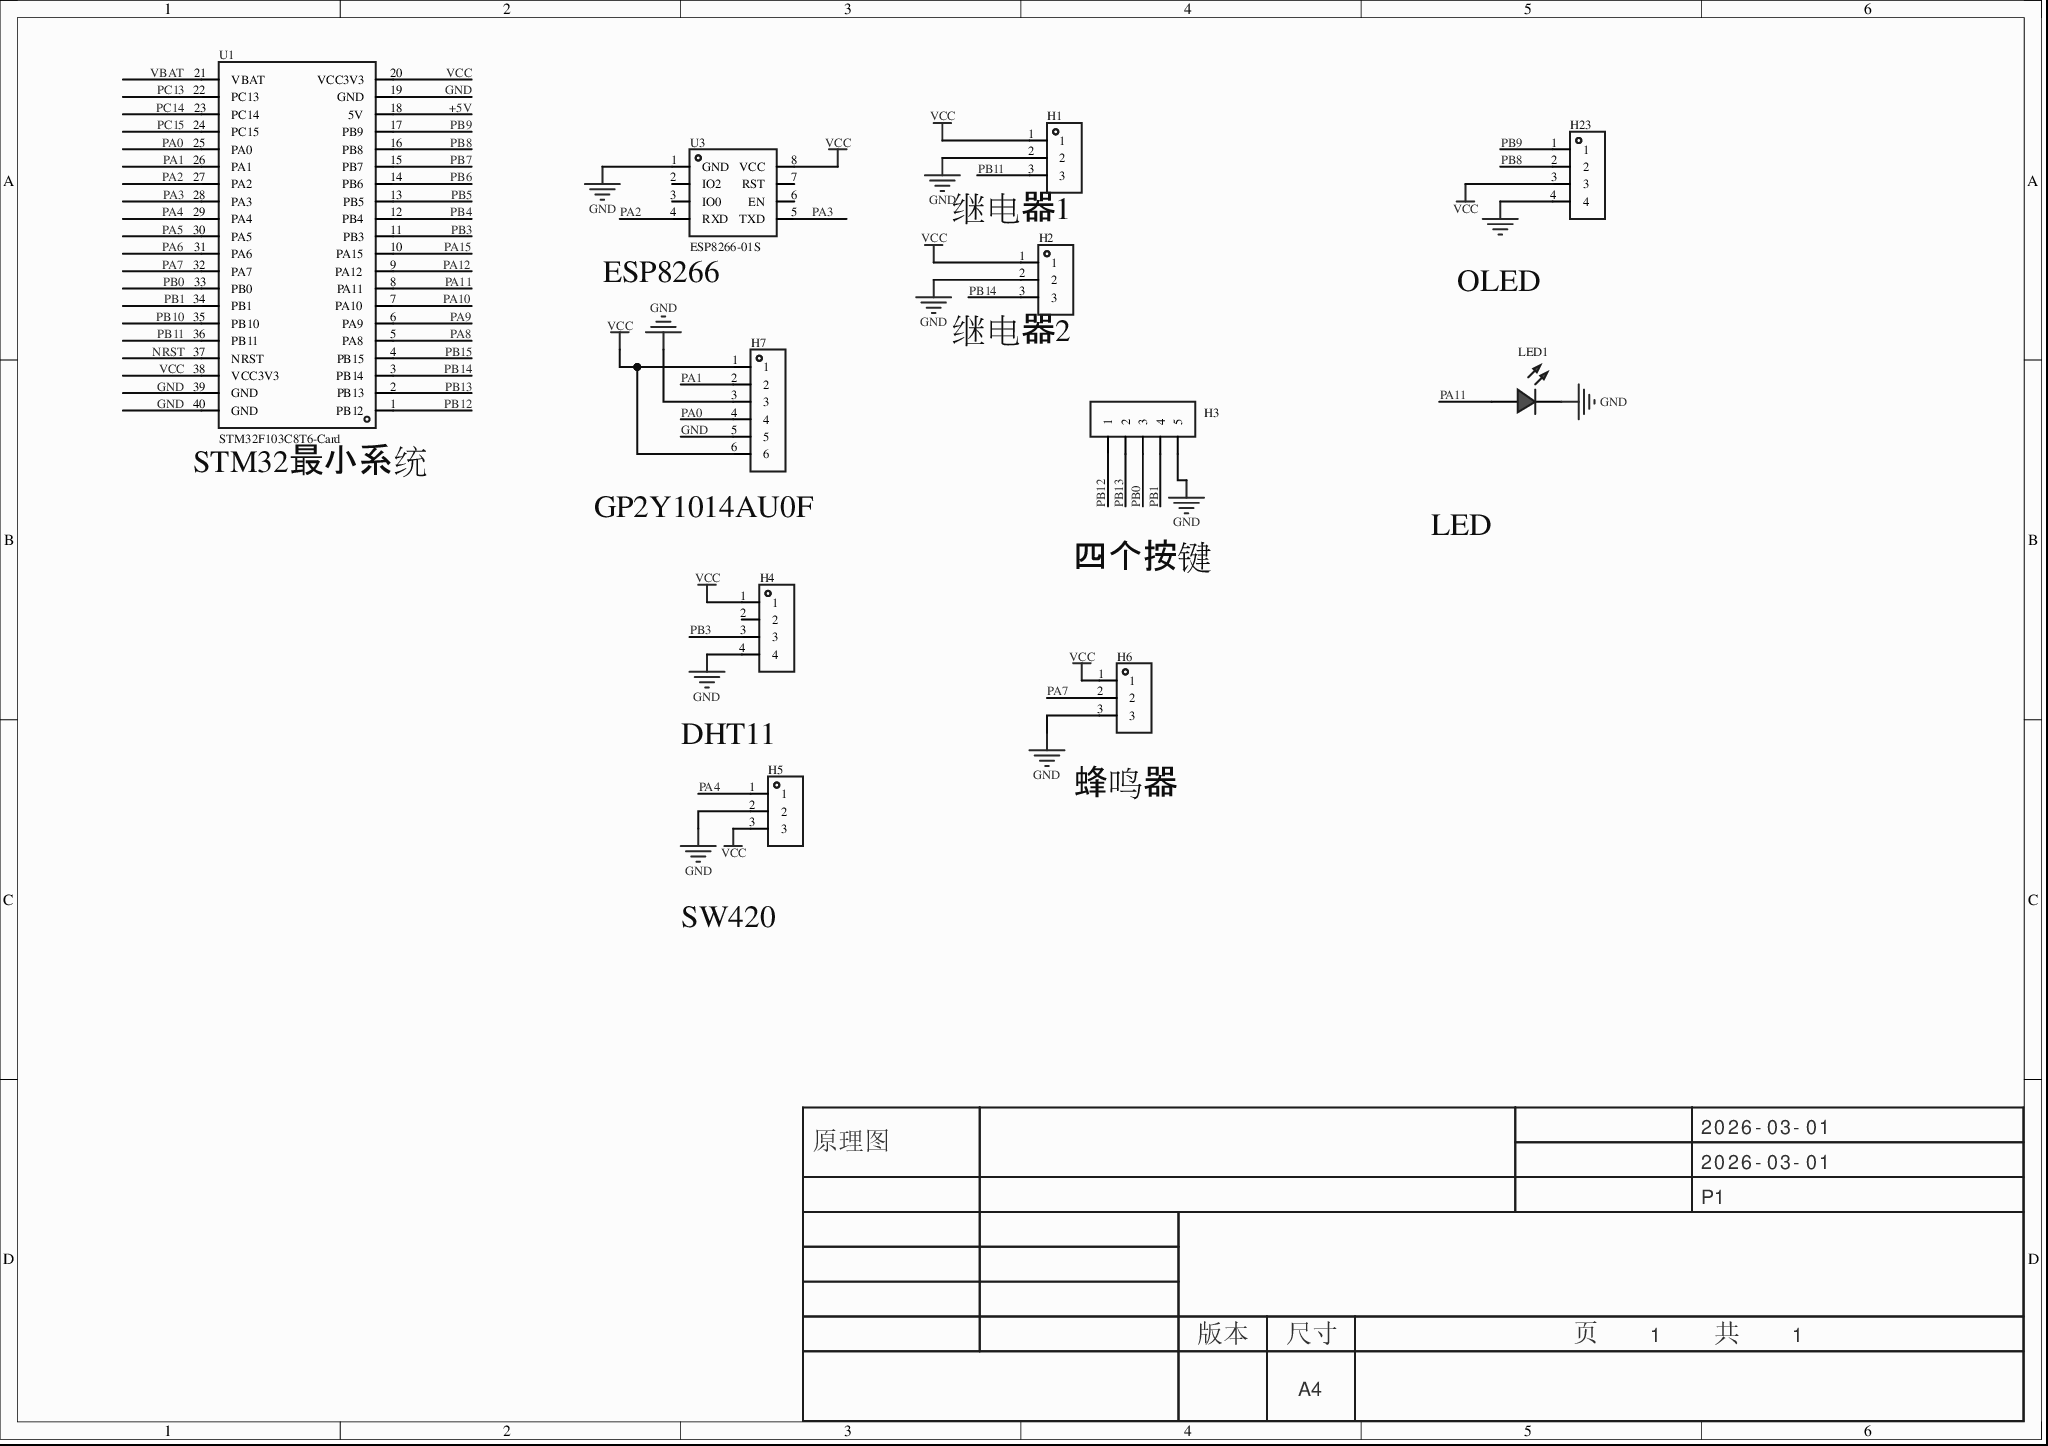
[diagram p0: MISC51358-3.schdoc]
# Altium project MISC51358-2.PrjPcb
1 sheet, 11 parts. Net scope: global (net labels, ports and power ports of the same name join across sheets).
Board file: MISC51358.pcbdoc

## Sheet MISC51358-3.schdoc
size 297 x 209 mm; Version: V1.0; @Project Name: MISC51358; @Page Count: 1; @Update Date: 2026-03-01; @Create Date: 2026-03-01; @Schematic Name: MISC51358; @Page No: 1; @Create Time: 18:58:15; @Update Time: 22:44:58; @Board Name: MISC51358

### Parts
H1  (no value)  [HDR-TH_3P-P2.54-V-F]
H2  (no value)  [HDR-TH_3P-P2.54-V-F]
H3  (no value)  [HDR-TH_5P-P2.54-V-F]
H4  (no value)  [HDR-TH_4P-P2.54-V-F]
H5  (no value)  [HDR-TH_3P-P2.54-V-F]
H6  (no value)  [HDR-TH_3P-P2.54-V-F]
H7  (no value)  [HDR-TH_6P-P2.54-V-F]
H23  (no value)  [HDR-TH_4P-P2.54-V-F]
LED1  (no value)  [LED_TH-3mm]
U1  STM32F103C8T6-Card  [CONN-TH_L53.3-W22.9_STM32F103C8T6-CARD]
U3  ESP8266-01S  [WIFIM-TH_ESP8266-01S]

### Nets
GND: H1.2 H2.2 H3.5 H4.4 H5.2 H6.3 H7.3 H7.5 H23.4 LED1.2(A) U1.19(GND) U1.39(GND) U1.40(GND) U3.1(GND)
VCC: H1.1 H2.1 H4.1 H5.3 H6.1 H7.1 H7.6 H23.3 U1.20(VCC3V3) U1.38(VCC3V3) U3.8(VCC)
+5V: U1.18(5V)
NRST: U1.37(NRST)
PA0: H7.4 U1.25(PA0)
PA1: H7.2 U1.26(PA1)
PA2: U1.27(PA2) U3.4(RXD)
PA3: U1.28(PA3) U3.5(TXD)
PA4: H5.1 U1.29(PA4)
PA5: U1.30(PA5)
PA6: U1.31(PA6)
PA7: H6.2 U1.32(PA7)
PA8: U1.5(PA8)
PA9: U1.6(PA9)
PA10: U1.7(PA10)
PA11: LED1.1(C) U1.8(PA11)
PA12: U1.9(PA12)
PA15: U1.10(PA15)
PB0: H3.3 U1.33(PB0)
PB1: H3.4 U1.34(PB1)
PB3: H4.3 U1.11(PB3)
PB4: U1.12(PB4)
PB5: U1.13(PB5)
PB6: U1.14(PB6)
PB7: U1.15(PB7)
PB8: H23.2 U1.16(PB8)
PB9: H23.1 U1.17(PB9)
PB10: U1.35(PB10)
PB11: H1.3 U1.36(PB11)
PB12: H3.1 U1.1(PB12)
PB13: H3.2 U1.2(PB13)
PB14: H2.3 U1.3(PB14)
PB15: U1.4(PB15)
PC13: U1.22(PC13)
PC14: U1.23(PC14)
PC15: U1.24(PC15)
VBAT: U1.21(VBAT)

Not connected (* = marked no-connect by the designer): H4 2*; U3 2(IO2) 3(IO0) 6(EN) 7(RST)

### Notes on the sheet
- 继电器1
- (near U3) ESP8266
- (near H2) 继电器2
- OLED
- (near U1) STM32最小系统
- (near H7) GP2Y1014AU0F
- 四个按键
- LED
- DHT11
- (near H6) 蜂鸣器
- SW420
- 2026-03-01
- 原理图
- P1
- 版本
- 尺寸
- A4
- 页    1    共    1

### Library data of the parts
H1 H2 H5 H6 = HDR-F_2.54_1x3P: Symbol: PM254V-11-03-H85; 3D Model: f3b3cc5aae9641bf9e56fc160cef875b; 3D Model Transform: 299.9994,100,0,0,0,0,0,0,-118.11; ConvertToPcb: yes; ModelName: HDR2.54-F-LI-1X3P; Device: HDR-F_2.54_1x3P; Supplier Part: C541850; Supplier Footprint: 插件; AddInBom: yes; FootprintName: HDR-TH_3P-P2.54-V-F
H3 = HDR-F_2.54_1x5P: Symbol: Header-Female-2.54_1x5; ConvertToPcb: yes; ModelId: f49cb6116a3d45e5a64915bf3e00773f; ModelTransform: 519.684,98.464,0,0,0,0,0,0,-124.016; Device: HDR-F_2.54_1x5P; AddInBom: yes; SupplierPart: C50950; Supplier Footprint: 插件; FootprintName: HDR-TH_5P-P2.54-V-F; ModelName: HDR-TH_5P-P2.54-V-F
H4 = HDR-F_2.54_1x4P: Symbol: 2.54-1*4P母; ConvertToPcb: yes; ModelId: d187812051054f85879fcaa51a310d8e0819f05c4eef4c71ace90d822a990e87; ModelTransform: 419.6842,98.464,0,0,0,0,0,0,-118.11; Device: HDR-F_2.54_1x4P; AddInBom: yes; SupplierPart: C2718488; Supplier Footprint: 插件; FootprintName: HDR-TH_4P-P2.54-V-F; ModelName: HDR-TH_4P-P2.54-V-F
H7 = HDR-F_2.54_1x6P: Symbol: Header-Female-2.54_1x6; 3D Model: 0f5bcf94dcda47d085f24cdca1696fe9; 3D Model Transform: 619.684,94.488,0,0,0,0,0,0,-125.984; ConvertToPcb: yes; Device: HDR-F_2.54_1x6P; Supplier Part: C40877; Supplier Footprint: 插件; AddInBom: yes; FootprintName: HDR-TH_6P-P2.54-V-F; ModelName: HDR-TH_6P-P2.54-V-F
H23 = HDR-F_2.54_1x4P: Symbol: 2.54-1*4P母; ConvertToPcb: yes; ModelId: d187812051054f85879fcaa51a310d8e; ModelTransform: 419.6842,98.464,0,0,0,0,0,0,-118.11; Device: HDR-F_2.54_1x4P; AddInBom: yes; SupplierPart: C2718488; Supplier Footprint: 插件; FootprintName: HDR-TH_4P-P2.54-V-F; ModelName: HDR-TH_4P-P2.54-V-F
LED1 = LED_TH-R_3mm: ConvertToPcb: yes; ModelId: a497c992633541038a38947cdc58012f0819f05c4eef4c71ace90d822a990e87; ModelName: LED-TH-3mm_R; ModelTransform: 141.274,153.327,0,0,0,0,-5.984,0,-137.795; Symbol: LED_TH-R; Device: LED_TH-R_3mm; AddInBom: yes; FootprintName: LED_TH-3mm; Supplier Footprint: 插件
U1 = STM32F103C8T6-Card: AddInBom: yes; Symbol: STM32F103C8T6-CARD; Device: STM32F103C8T6-Card; LCSC Part Name: STM32F103C8T6-Card; SupplierPart: C9900077949; ManufacturerPart: STM32F103C8T6-Card; Supplier Footprint: 插件; Supplier: LCSC; ConvertToPcb: yes; FootprintName: CONN-TH_L53.3-W22.9_STM32F103C8T6-CARD
U3 = ESP8266-01S: AddInBom: yes; ModelId: 7671a3a19d0d4245ae5d5806b59f4d510819f05c4eef4c71ace90d822a990e87; ModelTransform: 566.928,972.439,0,0,0,0,0,378.464,-118.11; Symbol: ESP8266-01S; Device: ESP8266-01S; LCSC Part Name: ESP8266-01S; SupplierPart: C9900150497; ManufacturerPart: ESP8266-01S; Supplier Footprint: TH-8P; JLCPCB Part Class: Extended Part; Supplier: LCSC; ConvertToPcb: yes; FootprintName: WIFIM-TH_ESP8266-01S; ModelName: WIFIM-TH_ESP8266-01S